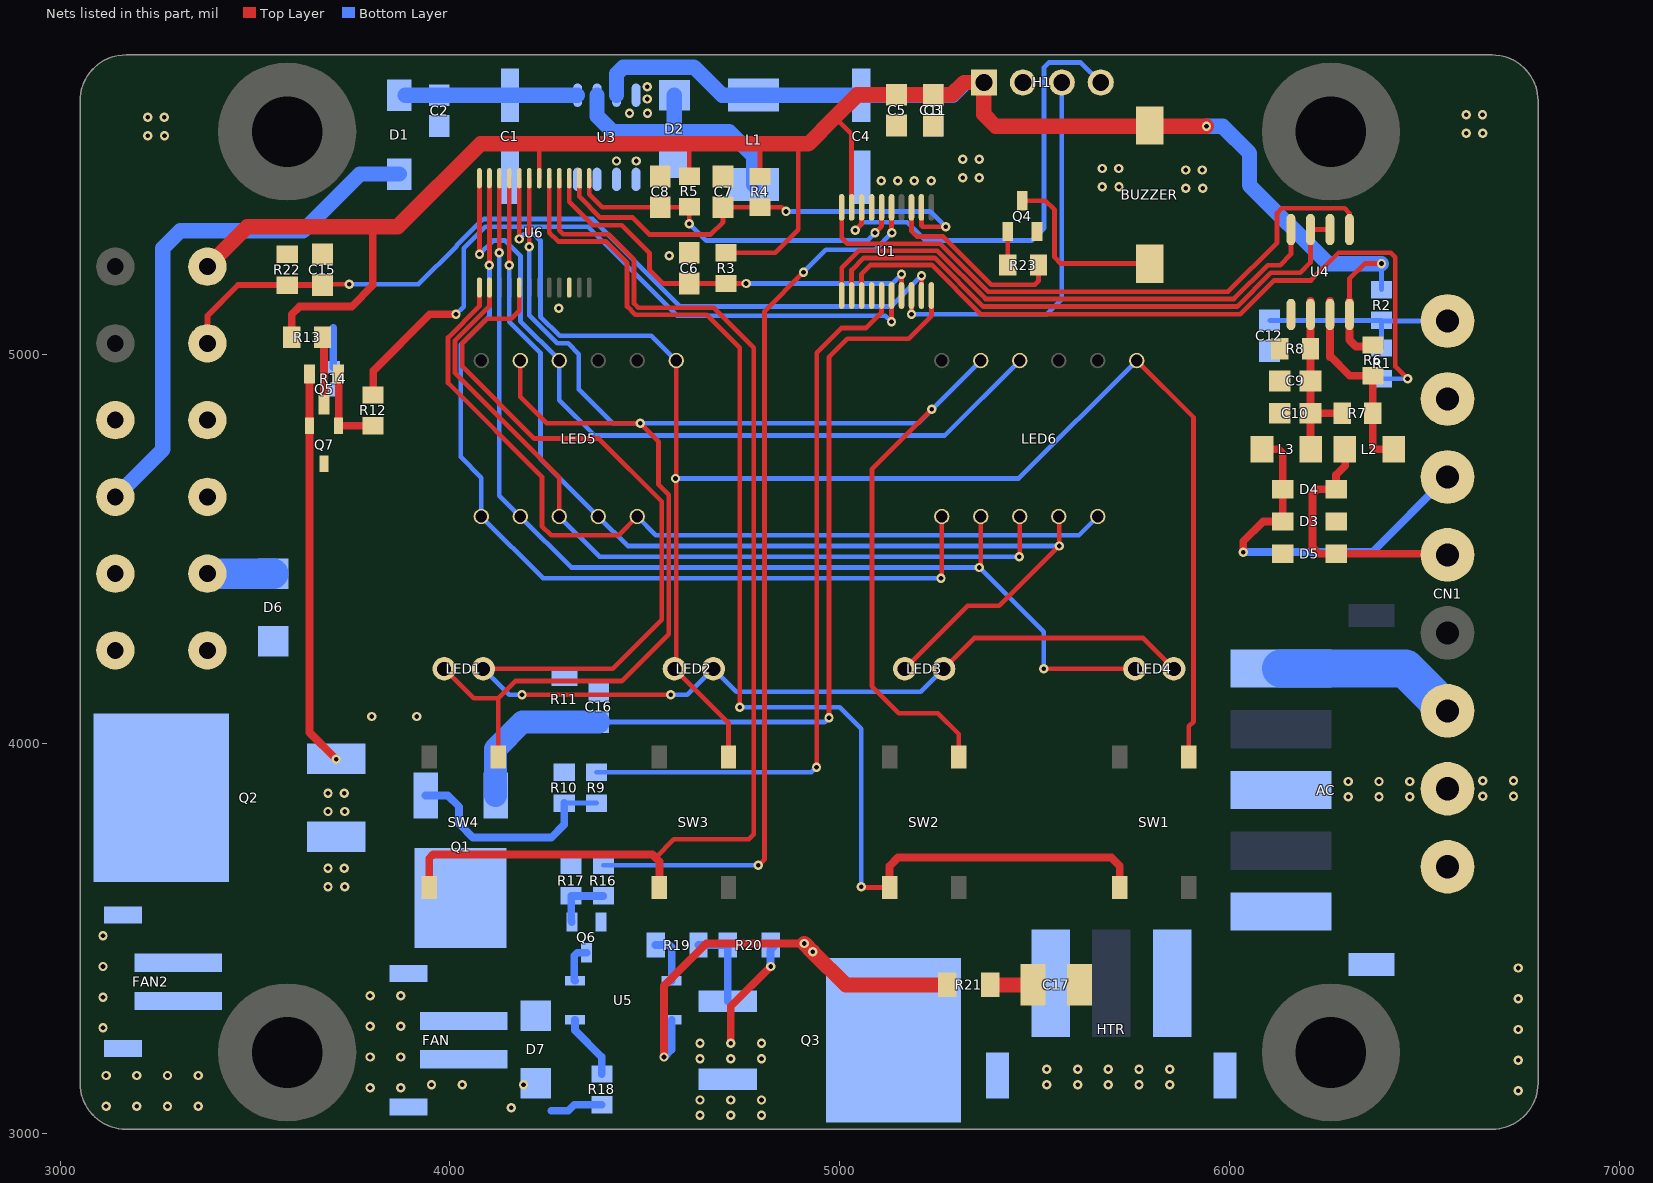
[diagram p0: the nets of this part, all layers, seen from the top]
# Altium PCB MISC84275.PcbDoc (part 2 of 3)
Units mil, origin at the board's own origin, x right, y up, seen from the top; angles counter-clockwise.
Board outline 3740.1 x 2755.9 mil, 2 copper layers (Top Layer, Bottom Layer), stack 62.2 mil thick; 76 components, 62 nets, 275 pads, 150 vias.

## Via types
v1: diameter 24, hole 12, Top Layer to Bottom Layer, 150 vias

## Nets (pads, with @x,y where several pads share a name; then routed paths per layer and width w, separated by ;. In a path a pad name is that pad's centre, name@x,y a point inside that pad or via, vN(x,y) a via of type N, cw(c..) or ccw(c..) an arc to the next point about the centre after c; other vN are vias at no path point) (continued)
7: LED1.2 LED2.2 LED3.2 LED4.2 U6.17 | length 3709.7
  Top Layer w12.1: LED1.2@4085.4,4192.9 4417.3,4192.9 4543.3,4318.9 4543.3,4622 4381.9,4783.5 4216.5,4783.5 4031.5,4968.5 4031.5,5027.6 4094.5,5090.6 4157.5,5090.6 4178.1,5111.2 U6.17@4178.1,5170.8 ; v1(4185,4126) v1(4566.9,4126) ; LED3.2@5266.5,4192.9 5345.3,4271.7 5778.3,4271.7 LED4.2@5857.1,4192.9
  Bottom Layer w12.1: LED1.2@4085.4,4192.9 4152.4,4126 v1(4185,4126) ; v1(4566.9,4126) 4609.1,4126 LED2.2@4676,4192.9 4735,4133.9 5207.5,4133.9 LED3.2@5266.5,4192.9
$1N7461: D2.1 L1.2 U3.2 | length 664.3
  Bottom Layer w39.4: U3.2@4377.5,5664.2 4377.5,5610.7 4417.3,5570.9 4576,5570.9 ; D2.1@4576,5664.2 4576,5570.9 ; L1.2@4779.1,5434.8 4779.1,5508.3 4716.5,5570.9 4576,5570.9
$1N14229: Q4.1 R23.2 | length 86.7
  Top Layer w12.1: R23.2@5431.1,5228.3 Q4.1@5431.1,5315
$1N14264: C9.2 C10.2 L3.1 R7.1 R8.2 U4.6 | length 458.9
  Top Layer w20: L3.1@6207.6,4759.5 C10.2@6207.6,4848.5 ; U4.6@6207.6,5137.2 R8.2@6207.6,5013.9 C9.2@6207.6,4931.2 C10.2@6207.6,4848.5 ; R7.1@6288.8,4848.5 C10.2@6207.6,4848.5
$1N14265: L2.1 R6.1 R7.2 U4.7 | length 519.1
  Top Layer w20: 6257.6,4991.8 6257.6,4995.8 ; U4.7@6257.6,5137.2 6257.6,4995.8 ; R6.1@6367.6,4948.8 R6.1@6367.6,4944.8 ; L2.1@6421,4755.9 6374,4755.9 6367.6,4762.4 R7.2@6367.6,4848.5 R6.1@6367.6,4944.8 ; 6257.6,4995.8 6308.5,4944.8 R6.1@6367.6,4944.8
$1N14291: BUZZER.2 Q4.3 | length 465
  Top Layer w12.1: Q4.3@5468.5,5393.7 5527.6,5393.7 5551.2,5370.1 5551.2,5248.3 5567.3,5232.3 BUZZER.2@5795.3,5232.3
$1N14293: R18.1 U5.1 | length 167.6
  Bottom Layer w19.7: U5.1@4320.9,3292.5 4320.9,3265.7 4389.8,3196.9 R18.1@4389.8,3153.5
$1N14295: Q3.3 R19.2 R20.1 | length 218.9
  Bottom Layer w19.7: R19.2@4637.8,3484.3 R20.1@4712.6,3484.3
  Bottom Layer w20: Q3.3@4712.6,3340.2 R20.1@4712.6,3484.3
$1N14296: R19.1 U5.3 | length 129.6
  Bottom Layer w19.7: R19.1@4527.6,3484.3 4563,3484.3 4568.9,3478.3 U5.3@4568.9,3392.5
$1N14298: C17.2 R21.1 | length 109.6
  Top Layer w39.4: R21.1@5385.8,3381.9 C17.2@5495.4,3381.9
$1N14301: Q6.1 R16.2 R17.1 | length 150.4
  Bottom Layer w19.7: Q6.1@4313,3543.3 4311,3545.3 R17.1@4311,3610.2 R16.2@4393.7,3610.2
$1N14303: Q6.3 U5.2 | length 99.8
  Bottom Layer w19.7: U5.2@4320.9,3392.5 4318.9,3394.5 4318.9,3456.7 4326.8,3464.6 Q6.3@4350.4,3464.6
$1N14304: Q5.1 Q7.1 R12.2 | length 221
  Top Layer w19.7: Q5.1@3714.6,4948.8 Q7.1@3714.6,4816.3 R12.2@3803.1,4816.3
$1N14306: Q2.1 Q5.2 Q7.2 | length 1016.7
  Top Layer w19.7: Q5.2@3639.8,4948.8 Q7.2@3639.8,4816.3 3639.8,4029.5 v1(3708.7,3960.6)
$1N14315: Q1.1 R9.2 R10.2 | length 577.5
  Bottom Layer w12.1: R10.2@4293.3,3848.4 R9.2@4376,3848.4
  Bottom Layer w20: Q1.1@3937.6,3867.8 3994.4,3867.8 4023.6,3838.6 4023.6,3795.3 4059.1,3759.8 4259.8,3759.8 4293.3,3793.3 R10.2@4293.3,3848.4
$1N14375: R1.1 U1.13 | length 1947.3
  Top Layer w12.1: U1.13@5056.1,5150.5 5056.1,5205.7 5079.2,5228.8 5235.8,5228.8 5362.2,5102.4 6027.6,5102.4 6114.2,5189 6208.7,5189 6279.5,5259.8 6413.4,5259.8 6425.2,5248 6425.2,4968.5 v1(6456.7,4937)
  Bottom Layer w12.1: R1.1@6389.8,4937 v1(6456.7,4937)
$1N14423: C1.1 C2.1 D1.1 U3.1 | length 441.7
  Bottom Layer w39.4: D1.1@3885.8,5664.2 C2.1@3972.7,5664.2 C1.1@4154.1,5664.2 U3.1@4327.5,5664.2
$1N14478: Q5.3 R13.1 | length 174.9
  Top Layer w19.7: R13.1@3673.2,5043.3 3677.2,5039.4 Q5.3@3677.2,4870.1
+5V: BUZZER.1 C3.2 C4.1 C5.1 C11.2 H1.1 L1.1 pad.0@3378,5224.4 R2.2 R3.2 R4.2 R5.2 R6.2 R13.2 U1.9 U3.3 U4.8 U6.6 | length 6315.6
  Top Layer w12.1: U6.6@4229.3,5451.3 4229.3,5537.8 4230.9,5539.4 ; R5.2@4614.2,5456.7 4614.2,5539.4 ; R3.2@4708.7,5259.8 4834.6,5259.8 4893.7,5318.9 4893.7,5539.4 ; R4.2@4795.3,5455.7 4795.3,5538.5 4796.2,5539.4 ; 4987.2,5607.3 5030.5,5564 U1.9@5030.5,5376.5 ; U4.8@6307.6,5137.2 6307.6,5193.4 6346.5,5232.3 v1(6389.8,5232.3)
  Top Layer w19.7: R13.2@3594.5,5043.3 3594.5,5102.4 3614.2,5122 3748,5122 3802.5,5176.5 3802.5,5326.8
  Top Layer w20: U4.8@6307.6,5137.2 6307.6,5117.5 6307.6,5036.3 6324.3,5019.6 R6.2@6367.6,5019.6
  Top Layer w39.4: pad.0@3378,5224.4 3480.3,5326.8 3802.5,5326.8 3866.1,5326.8 4078.7,5539.4 4230.9,5539.4 4614.2,5539.4 4796.2,5539.4 4893.7,5539.4 4919.3,5539.4 4987.2,5607.3 5045.3,5665.4 C5.1@5145.7,5665.4 C11.2@5240.2,5665.4 5287.4,5665.4 5318.9,5696.9 H1.1@5369.7,5696.9 5369.7,5614.6 5399.6,5584.6 v1(5940.9,5584.6)
  Bottom Layer w12.1: R2.2@6389.8,5165.4 v1(6389.8,5232.3)
  Bottom Layer w39.4: U3.3@4427.5,5664.2 4427.5,5718.9 4444.9,5736.2 4626,5736.2 4698,5664.2 L1.1@4779.1,5664.2 C4.1@5054.9,5664.2 5290.2,5664.2 5322.8,5696.9 H1.1@5369.7,5696.9 ; v1(5940.9,5584.6) 5982.3,5584.6 6051.2,5515.7 6051.2,5433.1 6252,5232.3 v1(6389.8,5232.3)
A: LED1.1 LED5.11 LED6.11 SW2.4 SW4.4 U6.7 | length 4676.5
  Top Layer w12.1: LED1.1@3985.4,4192.9 4060.9,4117.5 4124,4117.5 ; SW4.4@4124,3966.5 4124,4117.5 ; LED5.11@4180.7,4983.5 4180.7,4890.2 4248,4822.8 v1(4488.2,4822.8) 4535.4,4775.6 4535.4,4665.4 4561.4,4639.4 4561.4,4281.9 4440.9,4161.4 4168,4161.4 4124,4117.5 ; v1(4203.7,5275.6) U6.7@4203.7,5451.3 ; v1(5236.2,4858.3) 5082.7,4704.7 5082.7,4148 5152,4078.7 5252,4078.7 5305.1,4025.6 SW2.4@5305.1,3966.5
  Bottom Layer w12.1: v1(4203.7,5275.6) 4203.7,5099.4 4275.6,5027.6 4303.1,5027.6 4330.7,5000 4330.7,4909.4 4417.3,4822.8 v1(4488.2,4822.8) 5201.2,4822.8 LED6.11@5361.8,4983.5
AD: C15.2 pad.0@3378,5027.6 R22.2 U1.19 | length 2182.5
  Top Layer w12.1: C15.2@3673.2,5177.2 3675.2,5179.1 v1(3742.1,5179.1) ; U1.19@5209.7,5150.5 v1(5209.7,5200.8)
  Top Layer w15: pad.0@3378,5027.6 3378,5098.4 3456.7,5177.2 R22.2@3582.7,5177.2 C15.2@3673.2,5177.2
  Bottom Layer w12.1: v1(3742.1,5179.1) 3919.3,5179.1 4017.3,5277.1 4017.3,5279.2 4083,5344.9 4085.1,5344.9 4086.6,5346.5 4366.1,5346.5 4590.6,5122 5130.9,5122 v1(5209.7,5200.8)
AD5: C16.2 Q1.2 R11.2 U1.20 | length 2292.3
  Top Layer w12.1: v1(4972.4,4066.9) 4972.4,4992.1 5019.7,5039.4 5177.2,5039.4 5235.3,5097.5 U1.20@5235.3,5150.5
  Bottom Layer w12.1: C16.2@4381.7,4056.3 4961.8,4056.3 v1(4972.4,4066.9)
  Bottom Layer w59.1: Q1.2@4117.5,3867.8 4117.5,3987.6 4186.2,4056.3 R11.2@4293.6,4056.3 C16.2@4381.7,4056.3
B: LED2.1 LED5.7 LED6.7 SW1.4 SW3.4 U6.8 | length 4278.8
  Top Layer w12.1: v1(4178.1,5295.3) U6.8@4178.1,5451.3 ; LED5.7@4580.7,4983.5 4580.7,4197.6 LED2.1@4576,4192.9 4714.6,4054.3 SW3.4@4714.6,3966.5 ; LED6.7@5761.8,4983.5 5907.8,4837.5 5907.8,4057.4 5895.7,4045.3 SW1.4@5895.7,3966.5
  Bottom Layer w12.1: v1(4178.1,5295.3) 4190,5307.1 4216.5,5307.1 4232.3,5291.3 4232.3,5096.5 4281.5,5047.2 4516.9,5047.2 LED5.7@4580.7,4983.5 ; v1(4578.7,4681.1) 5459.4,4681.1 LED6.7@5761.8,4983.5
BUZZER: R23.1 U1.3 | length 488.4
  Top Layer w12.1: U1.3@5184.1,5376.5 5184.1,5315.9 5198.4,5301.6 5265.5,5301.6 5389.1,5178 5500.8,5178 5509.8,5187 R23.1@5509.8,5228.3
C: LED3.1 LED5.4 LED6.4 U6.9 | length 2778.9
  Top Layer w12.1: v1(4152.6,5228.3) U6.9@4152.6,5451.3 ; LED3.1@5166.5,4192.9 5328,4354.3 5409.4,4354.3 v1(5563,4507.9) 5563,4582.3 LED6.4@5561.8,4583.5
  Bottom Layer w12.1: v1(4152.6,5228.3) 4152.6,5083.7 4232.3,5003.9 4232.3,4731.9 LED5.4@4380.7,4583.5 4456.3,4507.9 v1(5563,4507.9)
CLK: C7.2 R4.1 U1.2 U6.2 | length 1209.4
  Top Layer w12.1: U6.2@4331.7,5451.3 4331.7,5404.5 4385.8,5350.4 4468.5,5350.4 4511.8,5307.1 4669.3,5307.1 4700.8,5338.6 C7.2@4700.8,5377 R4.1@4795.3,5377 4851.4,5377 v1(4862.2,5366.1) ; U1.2@5209.7,5376.5 5209.7,5329.7 5212.6,5326.8 v1(5271.7,5326.8)
  Bottom Layer w12.1: v1(4862.2,5366.1) 5232.3,5366.1 v1(5271.7,5326.8)
D: LED4.1 LED5.2 LED6.2 U6.10 | length 2815.8
  Top Layer w12.1: v1(4127,5259.8) U6.10@4127,5451.3 ; v1(5358.3,4452.8) 5361.8,4456.3 LED6.2@5361.8,4583.5 ; v1(5523.6,4192.9) LED4.1@5757.1,4192.9
  Bottom Layer w12.1: v1(4127,5259.8) 4127,4637.2 LED5.2@4180.7,4583.5 4311.4,4452.8 v1(5358.3,4452.8) 5523.6,4287.4 v1(5523.6,4192.9)
DIN: C8.2 R5.1 U1.6 U6.1 | length 930.3
  Top Layer w12.1: U6.1@4357.3,5451.3 4357.3,5410.4 4390.8,5377 C8.2@4539.4,5377 4613.2,5377 R5.1@4614.2,5378 v1(4614.2,5334.6) ; v1(5090.6,5311) 5107.3,5327.8 U1.6@5107.3,5376.5
  Bottom Layer w12.1: v1(4614.2,5334.6) 4657.5,5291.3 5070.9,5291.3 v1(5090.6,5311)
DP: LED5.3 LED6.3 U6.14 | length 2060.8
  Top Layer w12.1: U6.14@4101.4,5170.8 4101.4,5123.1 4013.4,5035.1 4013.4,4951.2 4280.7,4683.9 LED5.3@4280.7,4583.5 ; v1(5460.6,4480.3) 5461.8,4481.5 LED6.3@5461.8,4583.5
  Bottom Layer w12.1: LED5.3@4280.7,4583.5 4383.9,4480.3 v1(5460.6,4480.3)
E: LED5.1 LED6.1 U6.11 | length 2324.2
  Top Layer w12.1: v1(4101.4,5228.3) U6.11@4101.4,5451.3 ; v1(5259.8,4425.2) 5261.8,4427.2 LED6.1@5261.8,4583.5
  Bottom Layer w12.1: v1(4101.4,5228.3) 4101.4,5097.4 4027.6,5023.6 4027.6,4736.2 4080.7,4683.1 LED5.1@4080.7,4583.5 4239,4425.2 v1(5259.8,4425.2)
ES485-A: CN1.3 D3.1 D4.1 L3.2 | length 986.3
  Top Layer w20: v1(6035.4,4492.1) 6035.4,4519.7 6086.6,4570.9 D3.1@6136.7,4570.9 ; L3.2@6083,4755.9 6126,4755.9 6136.7,4745.2 D4.1@6136.7,4653.5 D3.1@6136.7,4570.8
  Bottom Layer w20: v1(6035.4,4492.1) 6366.1,4492.1 CN1.3@6559.1,4685.1
ES485-B: CN1.4 D4.2 D5.1 L2.2 | length 666
  Top Layer w20: L2.2@6296.7,4752.2 6296.7,4714 6273.3,4690.6 D4.2@6273.3,4653.5 6224.4,4653.5 6212.6,4641.7 6212.6,4503.9 6228.4,4488.1 D5.1@6273.3,4488.1 6556,4488.1 CN1.4@6559.1,4485.1
F: LED5.10 LED6.10 U6.12 | length 2041.1
  Top Layer w12.1: v1(4075.8,5255.9) U6.12@4075.8,5451.3
  Bottom Layer w12.1: v1(4075.8,5255.9) 4111.2,5291.3 4141.7,5291.3 4181.1,5252 4181.1,5084.7 4280.7,4985.1 LED5.10@4280.7,4983.5 4280.7,4882.2 4371.6,4791.3 5269.7,4791.3 LED6.10@5461.8,4983.5
FAN: R9.1 U1.15 | length 1886.1
  Top Layer w12.1: v1(4940.5,3940.3) 4940.9,3940.7 4940.9,5003.9 5003.9,5066.9 5066.9,5066.9 5107.3,5107.3 U1.15@5107.3,5150.5
  Bottom Layer w12.1: R9.1@4376,3927.2 4927.4,3927.2 v1(4940.5,3940.3)
FAN1: D7.2 FAN2.1 FAN.1 Q1.3
G: LED5.5 LED6.5 U6.13 | length 2240.2
  Top Layer w12.1: U6.13@4075.8,5170.8 4075.8,5123.1 3995.2,5042.6 3995.2,4926 4236.2,4685 4236.2,4559.1 4259.8,4535.4 4432.7,4535.4 LED5.5@4480.7,4583.5
  Bottom Layer w12.1: LED5.5@4480.7,4583.5 4528.7,4535.4 5613.8,4535.4 LED6.5@5661.8,4583.5
GND: C1.2 C2.2 C3.1 C4.2 C5.2 C6.1 C7.1 C8.1 C9.1 C10.1 C11.1 C12.2 C15.1 CN1.2 D2.2 D3.2 D5.2 H1.2 Q4.2 R8.1 R14.2 R22.1 U1.7 U3.4 U3.5 U3.6 U3.7 U3.8 U4.5 U6.22 | length 100.2
  Bottom Layer w20: R14.2@3700.8,4966.7 3700.8,5066.9
  other v1: 4279.5,5118.1 4562.4,5252 5888,5425.2 5930.9,5425.2 5673.7,5429.1 5716.5,5429.1 5106.3,5444.9 5148.5,5444.9 5191.6,5444.9 5234.5,5444.9 5315.4,5452.8 5358.3,5452.8 5888,5472.4 5930.2,5472.4 5673.7,5476.4 5715.9,5476.4 4427.5,5495.5 4478.1,5495.5 5315.4,5500 5357.6,5500 3225.2,5560.1 3268,5560.1 6606.8,5566.9 6649.6,5566.9 3225.2,5607.4 3267.4,5607.4 6606.8,5614.2 6649,5614.2 4460.6,5618.1 4506.8,5618.1 4506.3,5654.4 4506.3,5685.9
GND1: C16.1 pad.0@3141.7,4830.7 pad.0@3378,4830.7 Q2.3 Q6.2 Q7.3 R10.1 R11.1 R14.1 R17.2
  other v1: 3687.2,3633.9 3730.1,3633.9 3687.2,3681.1 3729.4,3681.1 3687.2,3826.8 3730.1,3826.8 3687.2,3874 3729.4,3874 3799.2,4070.3 3914.7,4070.3
HTR: R16.1 U1.5 | length 2306.8
  Top Layer w12.1: v1@4787.4,3685 4807.1,3704.7 4807.1,5110.2 v1(4907,5210.1) ; U1.5@5132.9,5376.5 5132.9,5312 v1(5133.9,5311)
  Bottom Layer w12.1: R16.1@4393.7,3689 v1(4791.3,3689) ; v1(4907,5210.1) 4964.6,5267.7 5090.6,5267.7 v1(5133.9,5311)
HTR1: HTR.3 Q3.2 R21.2 U5.4 | length 1102.1
  Top Layer w20: v1(4549.2,3196.9) 4549.2,3379.9 4657.5,3488.2 v1(4909.4,3488.2)
  Top Layer w39.4: v1(4909.4,3488.2) v1(4930.8,3466.8) 5015.7,3381.9 R21.2@5275.6,3381.9
  Bottom Layer w19.7: v1(4549.2,3196.9) 4568.9,3216.5 U5.4@4568.9,3292.5
KEY1: SW3.1 SW4.1 U6.4 | length 3090.7
  Top Layer w12.1: U6.4@4280.5,5451.3 4280.5,5317.9 4291.3,5307.2 4407.6,5307.2 4472.5,5242.3 4472.5,5129.9 4483.5,5118.9 4676.3,5118.9 4779.2,5016.1 4779.2,3768 4767.1,3755.9 4574.8,3755.9 4527.6,3708.7
  Top Layer w20: SW4.1@3946.9,3631.9 3946.9,3706.7 3956.7,3716.5 4519.7,3716.5 4527.6,3708.7 4537.4,3698.8 SW3.1@4537.4,3631.9
KEY2: SW1.1 SW2.1 U6.5 | length 3270.3
  Top Layer w12.1: U6.5@4254.9,5451.3 4254.9,5312 4277.9,5289 4400.1,5289 4454.4,5234.8 4454.4,5122.4 4476,5100.8 4659,5100.8 4743.7,5016.2 v1(4743.7,4094.5) ; v1(5055.1,3633.9) 5057.1,3631.9 SW2.1@5128,3631.9
  Top Layer w20: SW2.1@5128,3631.9 5128,3687 5149.6,3708.7 5696.9,3708.7 5718.5,3687 SW1.1@5718.5,3631.9
  Bottom Layer w12.1: v1(4743.7,4094.5) 5000,4094.5 5055.1,4039.4 v1(5055.1,3633.9)
L: AC.5 AC.7 CN1.8 HTR.1
  other v1: 6740.2,3110.2 6740.2,3189 6740.2,3267.7 6740.2,3346.5 6740.2,3425.2
N: AC.3 C17.1 CN1.7 HTR.4 HTR.5 Q3.1 R20.2 | length 293.6
  Top Layer w20: v1(4720.5,3232.3) 4720.5,3326.8 v1(4822.8,3429.1)
  Bottom Layer w20: v1(4822.8,3429.1) 4822.8,3472.4 R20.2@4830.7,3480.3
  other v1: 4641.7,3047.2 4720.5,3047.2 4799.2,3047.2 4641.7,3086.6 4720.5,3086.6 4799.2,3086.6 5531.5,3126 5610.2,3126 5689,3126 5767.7,3126 5846.5,3126 5531.5,3165.4 5610.2,3165.4 5689,3165.4 5767.7,3165.4 5846.5,3165.4 4641.7,3192.9 4720.5,3192.9 4799.2,3192.9 4641.7,3232.3 4799.2,3232.3 6304.8,3864.6 6383.5,3864.6 6462.2,3864.6 6649.6,3866.1 6728.3,3866.1 6304.8,3903.9 6383.5,3903.9 6462.2,3903.9 6649.6,3905.5 6728.3,3905.5
P: R12.1 U1.16 | length 1801.2
  Top Layer w12.1: v1(5132.9,5082.7) U1.16@5132.9,5150.5
  Top Layer w19.7: R12.1@3803.1,4895.1 3803.1,4956.7 3948.8,5102.4 v1(4015.7,5102.4)
  Bottom Layer w12.1: v1(4015.7,5102.4) 4035.4,5122 4035.4,5271.7 4090.6,5326.8 4354.3,5326.8 4582.7,5098.4 5117.1,5098.4 v1(5132.9,5082.7)
PGND: AC.1 CN1.6 | length 472.2
  Bottom Layer w98.4: AC.1@6131.9,4193.7 6450.5,4193.7 CN1.6@6559.1,4085.1
PL: D6.2 pad.0@3141.7,4240.2 pad.0@3378,4240.2 Q2.4
RD: U1.12 U4.2 U4.3 | length 1488.3
  Top Layer w12.1: U1.12@5030.5,5150.5 5030.5,5215.6 5061.9,5246.9 5243.3,5246.9 5368.2,5122 6019.4,5122 6106,5208.7 6181.1,5208.7 6207.6,5235.1 U4.3@6207.6,5319.7 U4.2@6257.6,5319.7
RXD: U1.10 U4.1 | length 1618.5
  Top Layer w12.1: U1.10@5004.9,5376.5 5004.9,5298.2 5019.7,5283.5 5258,5283.5 5381.6,5159.9 5996,5159.9 6122,5285.9 6122,5361.9 6134.2,5374 6295.3,5374 6307.6,5361.7 U4.1@6307.6,5319.7
SCL: U1.14
SDA: C12.1 CN1.1 R1.2 R2.1 | length 527.7
  Bottom Layer w12.1: C12.1@6102.8,5086.1 6388.8,5086.1 R2.1@6389.4,5086.8 ; R1.2@6389.8,5015.7 R2.1@6389.8,5086.6 6391.3,5085.1 CN1.1@6559.1,5085.1
STB: C6.2 R3.1 U1.17 U6.3 | length 1089.2
  Top Layer w12.1: U6.3@4306.1,5451.3 4306.1,5390.7 4366.1,5330.7 4440.9,5330.7 4511.8,5259.8 4511.8,5216.5 4547.2,5181.1 C6.2@4614.2,5181.1 R3.1@4708.7,5181.1 v1(4759.8,5181.1) ; U1.17@5158.5,5150.5 v1(5158.5,5204.7)
  Bottom Layer w12.1: v1(4759.8,5181.1) 5134.9,5181.1 v1(5158.5,5204.7)
SWCLK: H1.3 U1.18 | length 1005.8
  Top Layer w12.1: v1(5184.1,5102.4) U1.18@5184.1,5150.5
  Bottom Layer w12.1: v1(5184.1,5102.4) 5531.5,5102.4 5569.7,5140.6 H1.3@5569.7,5696.9
SWDIO: H1.4 U1.8 | length 1175.1
  Top Layer w12.1: v1(5039.7,5318.2) 5056.1,5334.6 U1.8@5056.1,5376.5
  Bottom Layer w12.1: v1(5039.7,5318.2) 5060.1,5338.6 5173.2,5338.6 5220.5,5291.3 5492.1,5291.3 5524.2,5323.4 5524.2,5735.9 5536.3,5748 5618.5,5748 H1.4@5669.7,5696.9
TXD: U1.11 U4.4 | length 1403.8
  Top Layer w12.1: U1.11@5004.9,5150.5 5004.9,5221.5 5048.5,5265 5250.8,5265 5374.1,5141.7 6011.3,5141.7 6097.9,5228.3 6129.9,5228.3 6157.6,5256 U4.4@6157.6,5319.7
VCC: D1.2 D6.1 D7.1 FAN2.2 FAN2.3 FAN2.4 FAN.2 FAN.3 FAN.4 pad.0@3141.7,4437 pad.0@3141.7,4633.9 pad.0@3378,4437 pad.0@3378,4633.9 R18.2 | length 1679.2
  Bottom Layer w19.7: 4259.8,3059.1 4303.1,3059.1 4318.9,3074.8 R18.2@4389.8,3074.8
  Bottom Layer w39.4: pad.0@3141.7,4633.9 3263.8,4755.9 3263.8,5271.7 3308.3,5316.1 3623.2,5316.1 3769.1,5462 D1.2@3870.1,5462
  Bottom Layer w78.7: pad.0@3378,4437 D6.1@3547.2,4437
  other v1: 4157.5,3066.9 3118.1,3070.9 3196.9,3070.9 3275.6,3070.9 3354.3,3070.9 3795.3,3118.1 3874,3118.1 3952.8,3126 4031.5,3126 4189,3126 3118.1,3149.6 3196.9,3149.6 3275.6,3149.6 3354.3,3149.6 3795.3,3196.9 3874,3196.9 3110.2,3271.7 3795.3,3275.6 3874,3275.6 3110.2,3350.4 3795.3,3354.3 3874,3354.3 3110.2,3429.1 3110.2,3507.9
pads on no net: AC.2 AC.4 AC.8 CN1.5 HTR.2 SW1.2 SW1.3 SW2.2 SW2.3 SW3.2 SW3.3 SW4.2 SW4.3 U1.1 U1.4 U6.15 U6.16